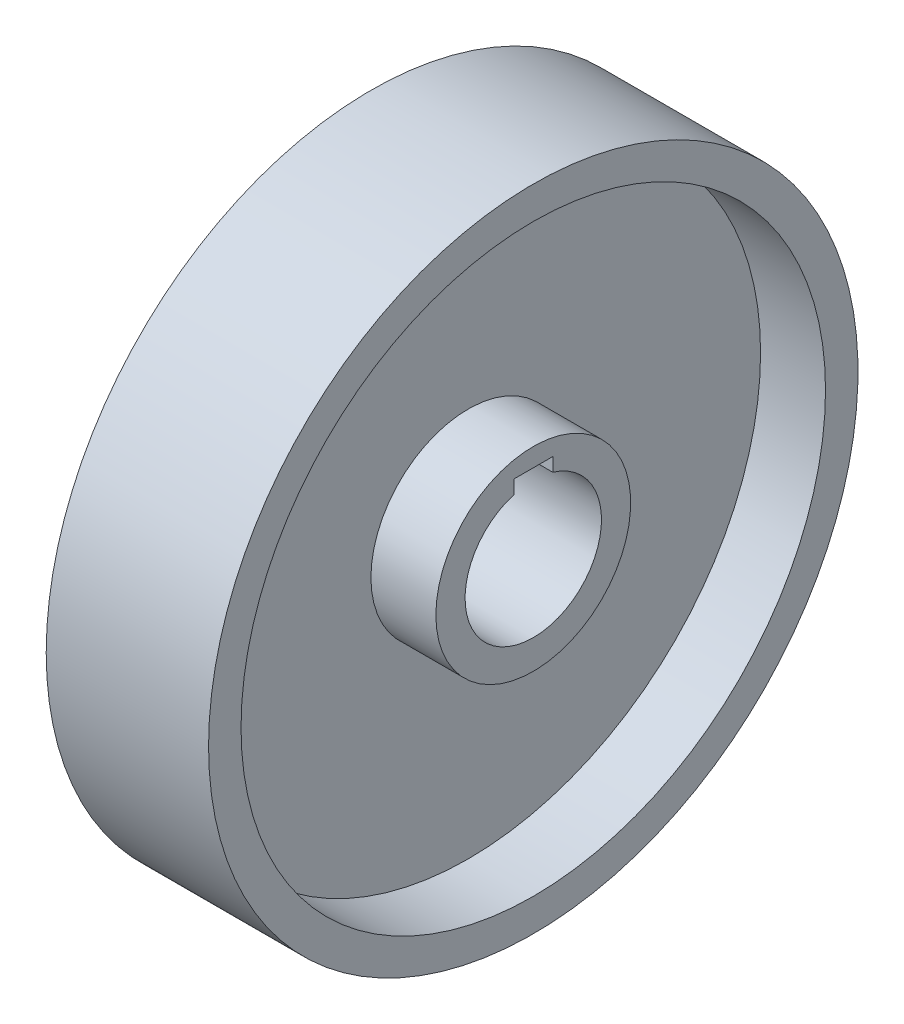
from build123d import *

# Parameters (mm, degrees)
CUT_EXTRUDE1_REACH = 152
SKETCH2_W          = 12
SKETCH2_H          = 6.6


with BuildPart() as part:
    # Sketch1 → Revolve1 (revolve)
    with BuildSketch(Plane.XY, mode=Mode.PRIVATE) as revolve1_sk:
        Polygon((-25, 21), (25, 21), (25, 30), (5, 30), (5, 90), (25, 90), (25, 100), (-25, 100), (-25, 90), (-5, 90), (-5, 30), (-25, 30), align=None)
    revolve(revolve1_sk.sketch.rotate(Axis((0, 0, 0), (1, 0, 0)), 90), axis=Axis((0, 0, 0), (1, 0, 0)))

    # Sketch2 → Cut-Extrude1 (cut, up to next)
    with BuildSketch(Plane(origin=(25, 0, 0), x_dir=(0, 0, -1), z_dir=(1, 0, 0)), mode=Mode.PRIVATE) as cut_extrude1_sk1:
        with Locations((0, 21)):
            Rectangle(SKETCH2_W, SKETCH2_H)
    cut_extrude1_tool1 = extrude(cut_extrude1_sk1.sketch, amount=-CUT_EXTRUDE1_REACH, mode=Mode.PRIVATE) & part.part
    add(cut_extrude1_tool1.solids().sort_by_distance((25, 21, 0))[0], mode=Mode.SUBTRACT)


solid = part.part
